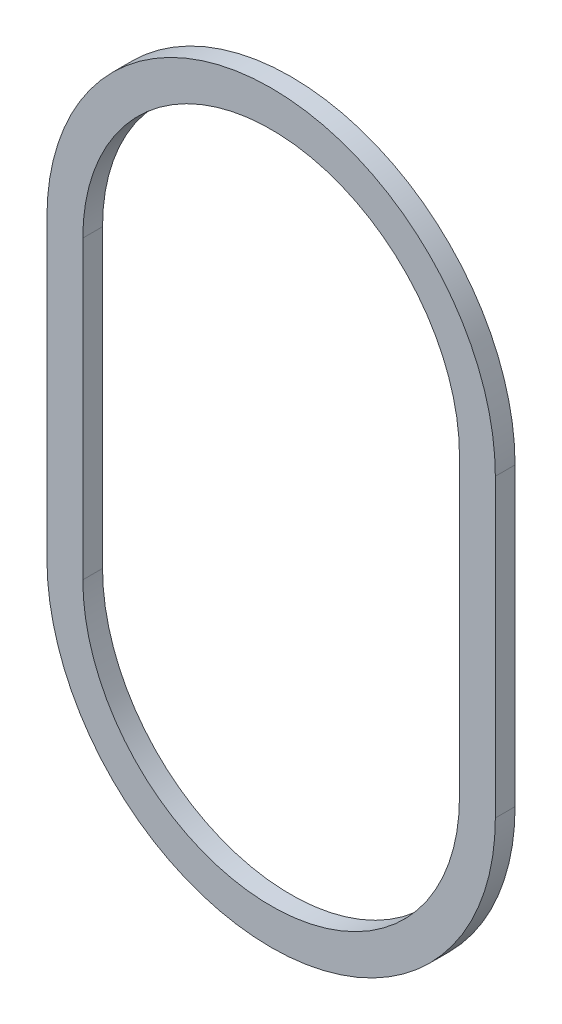
SolidWorks part; units mm, degrees
ref_plane "Front Plane" through (0, 0, 0) normal (0, 0, 1) x (1, 0, 0)
ref_plane "Top Plane" through (0, 0, 0) normal (0, 1, 0) x (1, 0, 0)
ref_plane "Right Plane" through (0, 0, 0) normal (1, 0, 0) x (0, 0, -1)
sketch "Sketch1" plane through (0, 0, 0) normal (0, 0, 1) x (1, 0, 0)
  line L0 (0, 0) -> (0, 33) construction
  line L1 (-21, 0) -> (-21, 33)
  line L8 (21, 0) -> (21, 33)
  line L9 (-25, 0) -> (-25, 33)
  line L10 (25, 0) -> (25, 33)
  arc A0 (-21, 0) -> (21, 0) centre (0, 0) ccw
  arc A1 (21, 33) -> (-21, 33) centre (0, 33) ccw
  arc A2 (25, 33) -> (-25, 33) centre (0, 33) ccw
  arc A3 (-25, 0) -> (25, 0) centre (0, 0) ccw
  point P2 (0, 16.5)
  dimension "D2" = 21
  dimension "D1" = 33
  dimension "D3" = 4
extrude "Boss-Extrude1" add sketch "Sketch1" along normal blind 2.2
